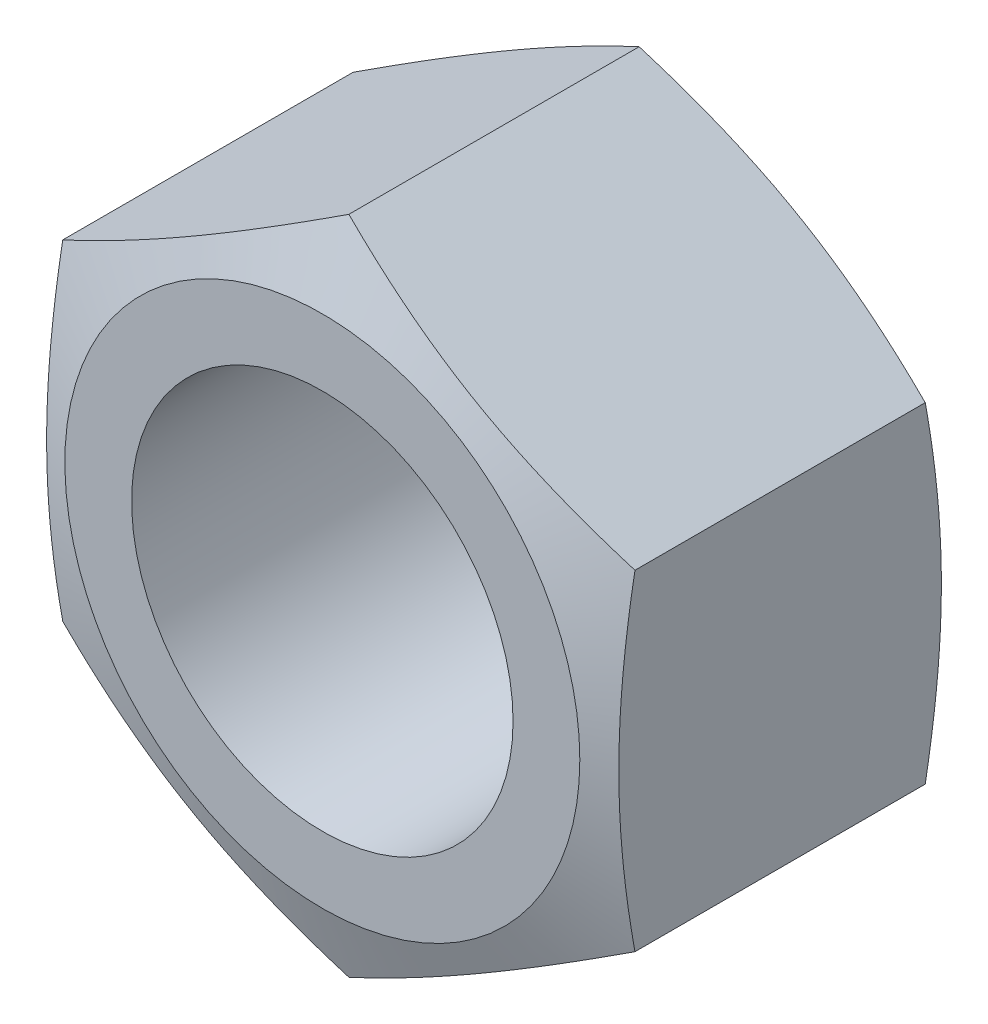
from build123d import *

# Parameters (mm, degrees)
BOSS_EXTRUDE1_DEPTH = 10.8
SKETCH5_R           = 6
CUT_EXTRUDE1_DEPTH  = 18.482562742


with BuildPart() as part:
    # Sketch1 → Boss-Extrude1 (new body)
    with BuildSketch(Plane.XY):
        Polygon((0, 10.392304845), (-9, 5.196152423), (-9, -5.196152423), (0, -10.392304845), (9, -5.196152423), (9, 5.196152423), align=None)
    extrude(amount=BOSS_EXTRUDE1_DEPTH)

    # Sketch4 → Cut-Revolve1 (revolve, cut)
    with BuildSketch(Plane(origin=(0, 0, 0), x_dir=(0, 0, -1), z_dir=(1, 0, 0)), mode=Mode.PRIVATE) as cut_revolve1_sk:
        Polygon((-10.8, -8.1), (-9.965669268, -10.392304845), (-10.8, -10.392304845), align=None)
    cut_revolve1 = revolve(cut_revolve1_sk.sketch.rotate(Axis((0, 0, 10.8), (0, 0, -1)), 119.999999988), axis=Axis((0, 0, 10.8), (0, 0, -1)), mode=Mode.SUBTRACT)

    # Mirror1: Cut-Revolve1 across plane
    add(cut_revolve1.mirror(Plane.XY.offset(5.4)), mode=Mode.SUBTRACT)

    # Sketch5 → Cut-Extrude1 (cut, through all)
    with BuildSketch(Plane.XY.offset(10.8)):
        Circle(SKETCH5_R)
    extrude(amount=-CUT_EXTRUDE1_DEPTH, mode=Mode.SUBTRACT)


solid = part.part
